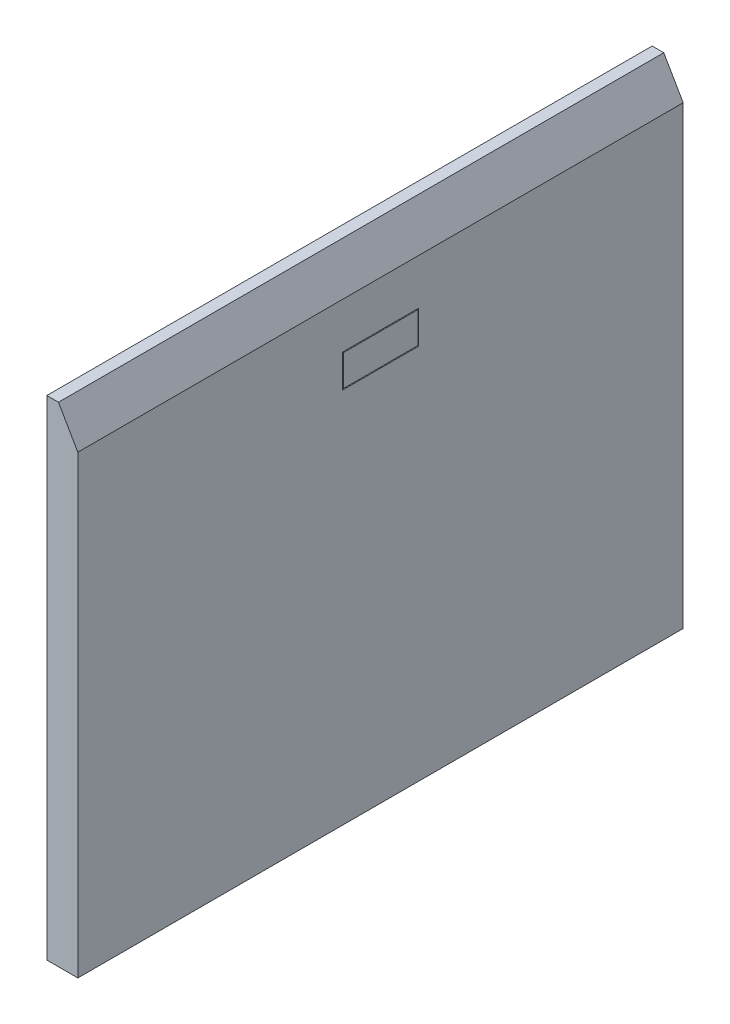
from build123d import *

# Parameters (mm, degrees)
BOSS_EXTRUDE1_DEPTH     = 780
SKETCH2_W               = 98.4
SKETCH2_H               = 42.4
SKETCH2_W_2             = 96
SKETCH2_H_2             = 40
CUT_EXTRUDE_THIN1_DEPTH = 2


with BuildPart() as part:
    # Sketch1 → Boss-Extrude1 (new body)
    with BuildSketch(Plane.XY):
        Polygon((0, 0), (0, -630), (40, -630), (40, -43.301270189), (15, 0), align=None)
    extrude(amount=BOSS_EXTRUDE1_DEPTH)

    # Sketch2 → Cut-Extrude-Thin1 (cut)
    with BuildSketch(Plane(origin=(40, 0, 0), x_dir=(0, 0, -1), z_dir=(1, 0, 0))):
        with Locations((-390, -123.301270189)):
            Rectangle(SKETCH2_W, SKETCH2_H)
        with Locations((-390, -123.301270189)):
            Rectangle(SKETCH2_W_2, SKETCH2_H_2, mode=Mode.SUBTRACT)
    extrude(amount=-CUT_EXTRUDE_THIN1_DEPTH, mode=Mode.SUBTRACT)


solid = part.part
